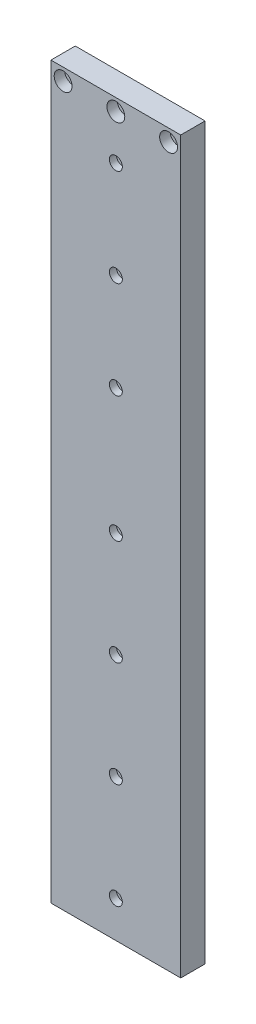
from build123d import *

# Parameters (mm, degrees)
SKETCH_1_W                   = 80
SKETCH_1_H                   = 450
EXTRUDE_1_DEPTH              = 15
HOLE_WIZARD_M6_1_D           = 6.6
HOLE_WIZARD_M6_1_CBORE_D     = 11
HOLE_WIZARD_M6_1_CBORE_DEPTH = 6.4
HOLE_WIZARD_M4_1_D           = 4.5
HOLE_WIZARD_M4_1_CBORE_D     = 8
HOLE_WIZARD_M4_1_CBORE_DEPTH = 4.4
HOLE_WIZARD_M4_2_D           = 4.5
HOLE_WIZARD_M4_2_CBORE_D     = 8
HOLE_WIZARD_M4_2_CBORE_DEPTH = 4.4
HOLE_WIZARD_M6_1_2_D         = 5
HOLE_WIZARD_M6_1_2_DEPTH     = 15
HOLE_WIZARD_M6_1_2_TIP       = 1.502151548


with BuildPart() as part:
    # 草图1 → 凸台-拉伸1 (new body)
    with BuildSketch(Plane.XY):
        Rectangle(SKETCH_1_W, SKETCH_1_H)
    extrude(amount=EXTRUDE_1_DEPTH)

    # Hole Wizard M6 _1 (through all)
    with Locations(Plane.XY.offset(15)):
        with Locations((-32.5, 217.5), (32.5, 217.5), (0, 217.5)):
            CounterBoreHole(HOLE_WIZARD_M6_1_D / 2, HOLE_WIZARD_M6_1_CBORE_D / 2, HOLE_WIZARD_M6_1_CBORE_DEPTH)

    # M4 六角凹头螺钉的柱形沉头孔1 (through all)
    with Locations(Plane.XY.offset(15)):
        with Locations((0, 190), (0, 130), (0, 70)):
            CounterBoreHole(HOLE_WIZARD_M4_1_D / 2, HOLE_WIZARD_M4_1_CBORE_D / 2, HOLE_WIZARD_M4_1_CBORE_DEPTH)

    # M4 六角凹头螺钉的柱形沉头孔2 (through all)
    with Locations(Plane.XY.offset(15)):
        with Locations((0, -202.5), (0, -137.5), (0, -72.5), (0, -7.5)):
            CounterBoreHole(HOLE_WIZARD_M4_2_D / 2, HOLE_WIZARD_M4_2_CBORE_D / 2, HOLE_WIZARD_M4_2_CBORE_DEPTH)

    # Hole Wizard M6 _1 2
    with Locations(Plane(origin=(0, -225, 0), x_dir=(-1, 0, 0), z_dir=(0, -1, 0))):
        with Locations((32.5, -7.5), (0, -7.5), (-32.5, -7.5)):
            Hole(HOLE_WIZARD_M6_1_2_D / 2, depth=HOLE_WIZARD_M6_1_2_DEPTH)
            with Locations((0, 0, -(HOLE_WIZARD_M6_1_2_DEPTH + HOLE_WIZARD_M6_1_2_TIP / 2))):  # 118° drill point
                Cone(0, HOLE_WIZARD_M6_1_2_D / 2, HOLE_WIZARD_M6_1_2_TIP, mode=Mode.SUBTRACT)


solid = part.part
